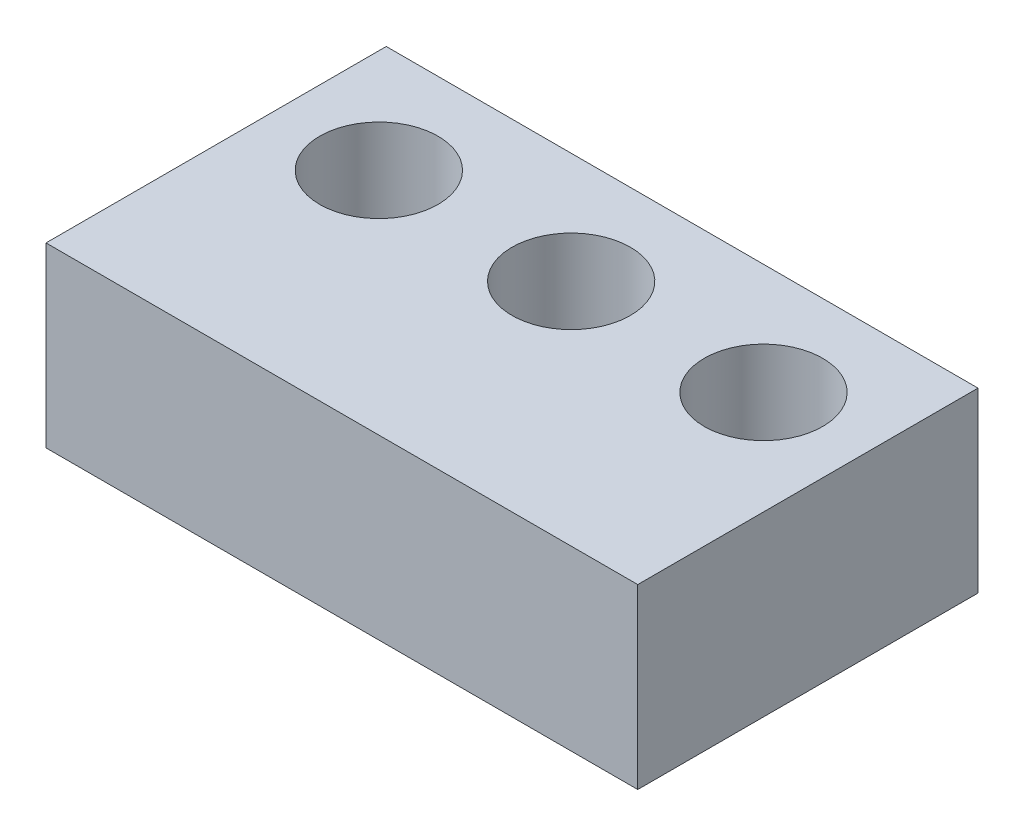
SolidWorks part; units mm, degrees
ref_plane "前视基准面" through (0, 0, 0) normal (0, 0, 1) x (1, 0, 0)
ref_plane "上视基准面" through (0, 0, 0) normal (0, 1, 0) x (1, 0, 0)
ref_plane "右视基准面" through (0, 0, 0) normal (1, 0, 0) x (0, 0, -1)
sketch "草图1" plane through (0, 0, 0) normal (0, 0, 1) x (1, 0, 0)
  line L1 (-20, -6) -> (20, -6)
  line L2 (-20, -6) -> (-20, 6)
  line L3 (-20, 6) -> (20, 6)
  line L4 (20, -6) -> (20, 6)
  line L5 (-20, -6) -> (20, 6) construction
  line L6 (-20, 6) -> (20, -6) construction
  point P0 (0, 0)
  dimension "D1" = 12
  dimension "D2" = 40
extrude "凸台-拉伸1" add sketch "草图1" along normal mid plane 15
sketch "草图2" plane through (0, 6, 0) normal (0, 1, 0) x (1, 0, 0)
  line L0 (-20, -7.5) -> (-20, 7.5) construction
  line L1 (20, -7.5) -> (20, 7.5) construction
  circle A0 centre (-13, 0) radius 4
  circle A1 centre (13, 0) radius 4
  point P4 (0, 0)
extrude "切除-拉伸1" cut sketch "草图2" against normal up to next
sketch "草图3" plane through (0, -6, 0) normal (0, -1, 0) x (1, 0, 0)
  circle A0 centre (0, 0) radius 4
  dimension "D1" = 8
extrude "切除-拉伸2" cut sketch "草图3" against normal up to next
sketch "草图4" plane through (0, 0, 7.5) normal (0, 0, 1) x (1, 0, 0)
  line L0 (20, -6) -> (20, 6) construction
  line L2 (-20, 6) -> (-20, -6) construction
  circle A0 centre (14.5, 0) radius 2.75
  circle A1 centre (-14.5, 0) radius 2.75
  dimension "D3" = 5.5
  dimension "D1" = 5.5
  dimension "D2" = 5.5
extrude "切除-拉伸3" [suppressed] cut sketch "草图4" against normal up to next
sketch "草图5" plane through (0, 0, 7.5) normal (0, 0, 1) x (1, 0, 0)
  line L0 (-20, 6) -> (-20, -6) construction
  line L5 (20, -6) -> (-20, -6)
  line L6 (20, -6) -> (20, 19)
  line L7 (20, 19) -> (-20, 19)
  line L8 (-20, -6) -> (-20, 19)
  dimension "D1" = 25
extrude "凸台-拉伸2" [suppressed] add sketch "草图5" along normal blind 6
sketch "草图6" plane through (0, 0, 7.5) normal (0, 0, 1) x (1, 0, 0)
  line L1 (-20, -6) -> (20, -6)
  line L2 (-20, -6) -> (-20, 6)
  line L3 (-20, 6) -> (20, 6)
  line L4 (20, -6) -> (20, 6)
extrude "凸台-拉伸3" add sketch "草图6" along normal blind 8
equation "\"D1@草图2\"=\"D2@草图2\""
